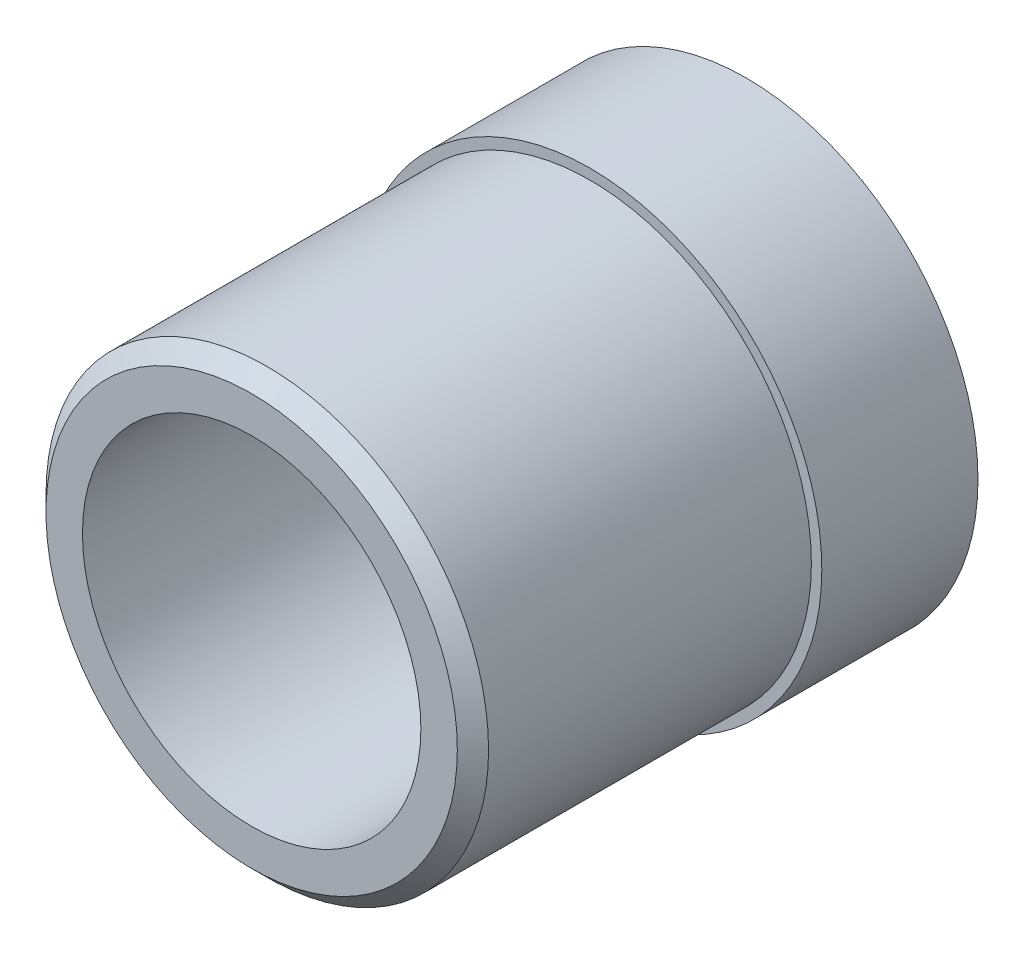
from build123d import *

# Parameters (mm, degrees)
SKETCH_1_R          = 44.5
SKETCH_1_R_2        = 32.5
EXTRUDE_1_DEPTH     = 95
CUT_EXTRUDE_START   = -65
SKETCH_2_R          = 44.5
SKETCH_2_R_2        = 42.5
CUT_EXTRUDE_1_DEPTH = 65
CHAMFER_1_SIZE      = 3


with BuildPart() as part:
    # 草图1 → 凸台-拉伸1 (new body)
    with BuildSketch(Plane.XY):
        Circle(SKETCH_1_R)
        Circle(SKETCH_1_R_2, mode=Mode.SUBTRACT)
    extrude(amount=EXTRUDE_1_DEPTH)

    # 草图2 → 切除-拉伸1 (cut)
    with BuildSketch(Plane.XY.offset(95).offset(CUT_EXTRUDE_START)):
        Circle(SKETCH_2_R)
        Circle(SKETCH_2_R_2, mode=Mode.SUBTRACT)
    extrude(amount=CUT_EXTRUDE_1_DEPTH, mode=Mode.SUBTRACT)

    # 倒角1
    chamfer_1_edges = [part.edges().sort_by_distance(p)[0] for p in [
        (-42.5, 0, 95),
    ]]
    chamfer(chamfer_1_edges, length=CHAMFER_1_SIZE)


solid = part.part
